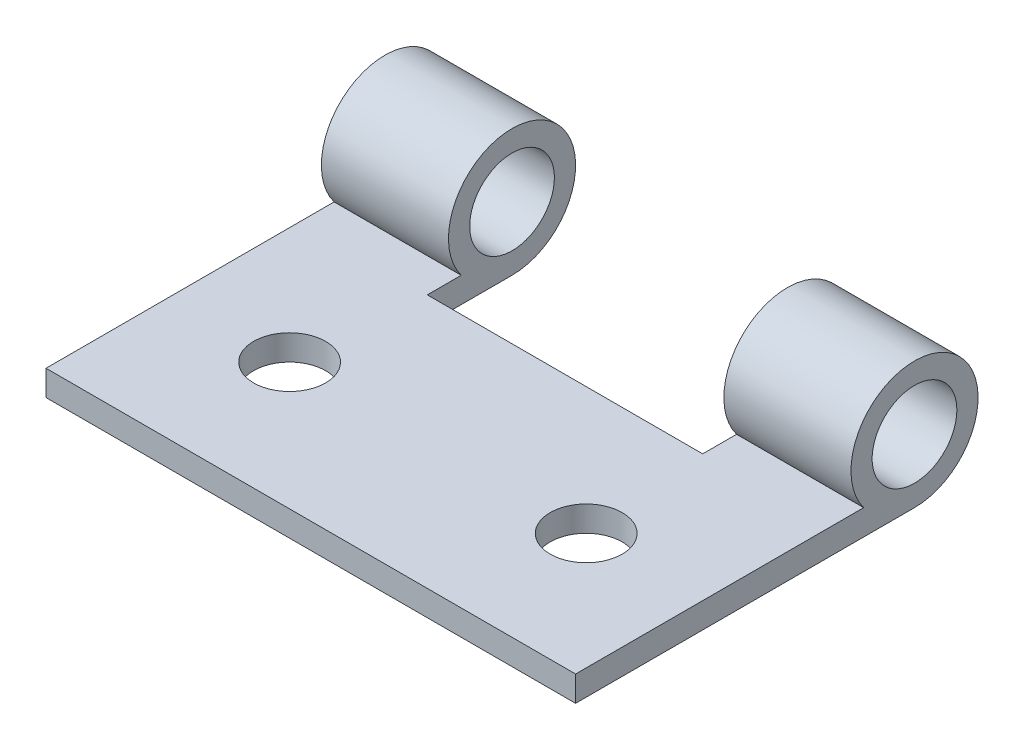
from build123d import *

# Parameters (mm, degrees)
SKETCH_1_R          = 2
EXTRUDE_1_DEPTH     = 12.5
SKETCH_2_R          = 1.7
CUT_EXTRUDE_1_DEPTH = 21.863604674
CUT_EXTRUDE_2_DEPTH = 6.5


with BuildPart() as part:
    # 草图1 → 凸台-拉伸1 (new, symmetric)
    with BuildSketch(Plane(origin=(0, 0, 0), x_dir=(0, 0, -1), z_dir=(1, 0, 0))):
        with BuildLine():
            Line((0, -3), (-16, -3))
            Line((-16, -3), (-16, -1.8))
            Line((-16, -1.8), (-2.4, -1.8))
            ThreePointArc((-2.4, -1.8), (1.341640786, 2.683281573), (0, -3))
        make_face()
        Circle(SKETCH_1_R, mode=Mode.SUBTRACT)
    extrude(amount=EXTRUDE_1_DEPTH, both=True)

    # 草图2 → 切除-拉伸1 (cut, through all)
    with BuildSketch(Plane(origin=(0, -1.8, 0), x_dir=(1, 0, 0), z_dir=(0, 1, 0))):
        with Locations(Location((-7, -10, 0), (0, 0, 270))):
            Circle(SKETCH_2_R)
        with Locations(Location((7, -10, 0), (0, 0, 270))):
            Circle(SKETCH_2_R)
    extrude(amount=-CUT_EXTRUDE_1_DEPTH, mode=Mode.SUBTRACT)

    # 草图3 → 切除-拉伸2 (cut, symmetric)
    with BuildSketch(Plane(origin=(0, 0, 0), x_dir=(0, 0, -1), z_dir=(1, 0, 0))):
        with BuildLine():
            Line((-4, -3), (0, -3))
            ThreePointArc((0, -3), (1.341640786, 2.683281573), (-2.4, -1.8))
            Line((-2.4, -1.8), (-4, -1.8))
            Line((-4, -1.8), (-4, -3))
        make_face()
    extrude(amount=CUT_EXTRUDE_2_DEPTH, both=True, mode=Mode.SUBTRACT)


solid = part.part
